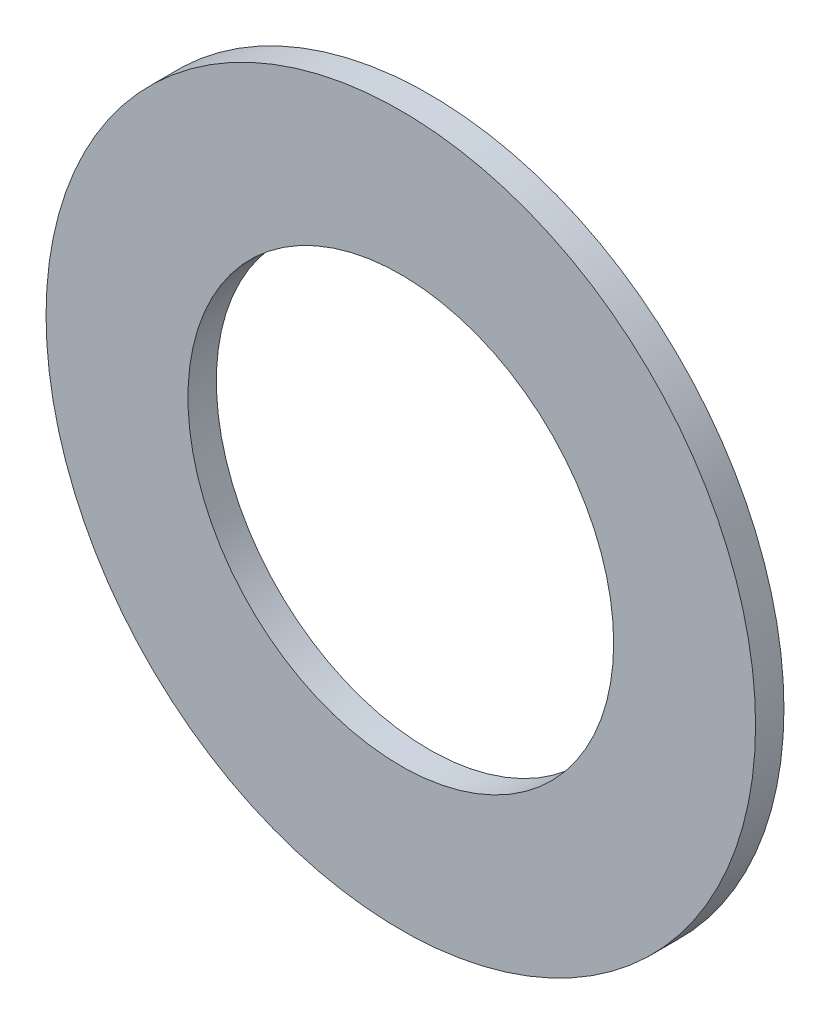
SolidWorks part; units mm, degrees
ref_plane "前视基准面" through (0, 0, 0) normal (0, 0, 1) x (1, 0, 0)
ref_plane "上视基准面" through (0, 0, 0) normal (0, 1, 0) x (1, 0, 0)
ref_plane "右视基准面" through (0, 0, 0) normal (1, 0, 0) x (0, 0, -1)
sketch "草图1" plane through (0, 0, 0) normal (0, 0, 1) x (1, 0, 0)
  circle A0 centre (-3.1504, -4.2341) radius 9
  circle A1 centre (-3.1504, -4.2341) radius 15
  dimension "D1" = 18
  dimension "D2" = 30
extrude "凸台-拉伸1" add sketch "草图1" along normal blind 1.2
